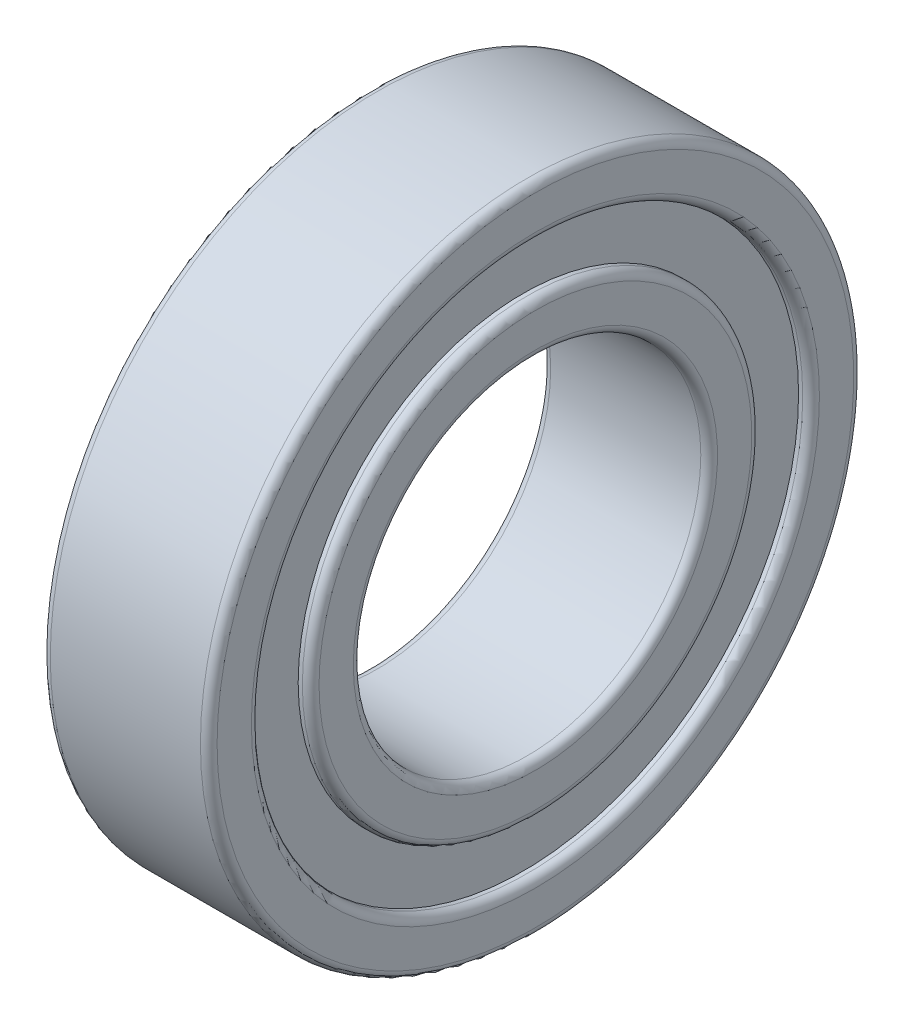
from build123d import *
from build123d.topology import SkipClean

# Parameters (mm, degrees)
SKETCH_5_W               = 1.65
SKETCH_5_H               = 1.1
PATTERN_CIRCULAR_5_COUNT = 16
PATTERN_CIRCULAR_2_COUNT = 16
SKETCH_8_W               = 0.6
SKETCH_8_H               = 4.866666666


with BuildPart() as part:
    # 草图2 → 旋转1 (revolve)
    with BuildSketch(Plane.XY, mode=Mode.PRIVATE) as revolve_1_sk:
        with BuildLine():
            Line((5.4, 12.5), (-5.4, 12.5))
            ThreePointArc((-5.4, 12.5), (-5.824264069, 12.675735931), (-6, 13.1))
            Line((-6, 13.1), (-6, 15.566666667))
            ThreePointArc((-6, 15.566666667), (-5.824264069, 15.990930735), (-5.4, 16.166666667))
            Line((-5.4, 16.166666667), (-2.049728979, 16.166666667))
            ThreePointArc((-2.049728979, 16.166666667), (0, 15.25), (2.049728979, 16.166666667))
            Line((2.049728979, 16.166666667), (5.4, 16.166666667))
            ThreePointArc((5.4, 16.166666667), (5.824264069, 15.990930735), (6, 15.566666667))
            Line((6, 15.566666667), (6, 13.1))
            ThreePointArc((6, 13.1), (5.824264069, 12.675735931), (5.4, 12.5))
        make_face()
        with BuildLine():
            Line((-6, 22.9), (-6, 20.433333333))
            ThreePointArc((-6, 20.433333333), (-5.824264069, 20.009069265), (-5.4, 19.833333333))
            Line((-5.4, 19.833333333), (-2.049728979, 19.833333333))
            ThreePointArc((-2.049728979, 19.833333333), (0, 20.75), (2.049728979, 19.833333333))
            Line((2.049728979, 19.833333333), (5.4, 19.833333333))
            ThreePointArc((5.4, 19.833333333), (5.824264069, 20.009069265), (6, 20.433333333))
            Line((6, 20.433333333), (6, 22.9))
            ThreePointArc((6, 22.9), (5.824264069, 23.324264069), (5.4, 23.5))
            Line((5.4, 23.5), (-5.4, 23.5))
            ThreePointArc((-5.4, 23.5), (-5.824264069, 23.324264069), (-6, 22.9))
        make_face()
    revolve(revolve_1_sk.sketch.rotate(Axis((-3.5, 0, 0), (1, 0, 0)), 90), axis=Axis((-3.5, 0, 0), (1, 0, 0)))


with BuildPart() as body_2:
    # 草图5 → 旋转3 (revolve)
    with BuildSketch(Plane.XY, mode=Mode.PRIVATE) as revolve_3_sk:
        with Locations((0, 18)):
            Rectangle(SKETCH_5_W, SKETCH_5_H)
    revolve(revolve_3_sk.sketch.rotate(Axis((-19.927092192, 0, 0), (1, 0, 0)), 90), axis=Axis((-19.927092192, 0, 0), (1, 0, 0)))



with BuildPart() as body_3:
    # 草图3 → 旋转2 (revolve)
    with BuildSketch(Plane.XY):
        with BuildLine():
            Line((-3.025, 18), (3.025, 18))
            ThreePointArc((3.025, 18), (0, 21.025), (-3.025, 18))
        make_face()
    revolve(axis=Axis((-3.025, 18, 0), (1, 0, 0)))


with BuildPart() as pattern_circular_5_1:
    # 阵列(圆周)5: pattern copy
    add(body_3.part.rotate(Axis((0, 0, 0), (1, 0, 0)), 1 * 360 / PATTERN_CIRCULAR_5_COUNT))


with BuildPart() as pattern_circular_5_2:
    # 阵列(圆周)5: pattern copy
    add(body_3.part.rotate(Axis((0, 0, 0), (1, 0, 0)), 2 * 360 / PATTERN_CIRCULAR_5_COUNT))


with BuildPart() as pattern_circular_5_3:
    # 阵列(圆周)5: pattern copy
    add(body_3.part.rotate(Axis((0, 0, 0), (1, 0, 0)), 3 * 360 / PATTERN_CIRCULAR_5_COUNT))


with BuildPart() as pattern_circular_5_4:
    # 阵列(圆周)5: pattern copy
    add(body_3.part.rotate(Axis((0, 0, 0), (1, 0, 0)), 4 * 360 / PATTERN_CIRCULAR_5_COUNT))


with BuildPart() as pattern_circular_5_5:
    # 阵列(圆周)5: pattern copy
    add(body_3.part.rotate(Axis((0, 0, 0), (1, 0, 0)), 5 * 360 / PATTERN_CIRCULAR_5_COUNT))


with BuildPart() as pattern_circular_5_6:
    # 阵列(圆周)5: pattern copy
    add(body_3.part.rotate(Axis((0, 0, 0), (1, 0, 0)), 6 * 360 / PATTERN_CIRCULAR_5_COUNT))


with BuildPart() as pattern_circular_5_7:
    # 阵列(圆周)5: pattern copy
    add(body_3.part.rotate(Axis((0, 0, 0), (1, 0, 0)), 7 * 360 / PATTERN_CIRCULAR_5_COUNT))


with BuildPart() as pattern_circular_5_8:
    # 阵列(圆周)5: pattern copy
    add(body_3.part.rotate(Axis((0, 0, 0), (1, 0, 0)), 8 * 360 / PATTERN_CIRCULAR_5_COUNT))


with BuildPart() as pattern_circular_5_9:
    # 阵列(圆周)5: pattern copy
    add(body_3.part.rotate(Axis((0, 0, 0), (1, 0, 0)), 9 * 360 / PATTERN_CIRCULAR_5_COUNT))


with BuildPart() as pattern_circular_5_10:
    # 阵列(圆周)5: pattern copy
    add(body_3.part.rotate(Axis((0, 0, 0), (1, 0, 0)), 10 * 360 / PATTERN_CIRCULAR_5_COUNT))


with BuildPart() as pattern_circular_5_11:
    # 阵列(圆周)5: pattern copy
    add(body_3.part.rotate(Axis((0, 0, 0), (1, 0, 0)), 11 * 360 / PATTERN_CIRCULAR_5_COUNT))


with BuildPart() as pattern_circular_5_12:
    # 阵列(圆周)5: pattern copy
    add(body_3.part.rotate(Axis((0, 0, 0), (1, 0, 0)), 12 * 360 / PATTERN_CIRCULAR_5_COUNT))


with BuildPart() as pattern_circular_5_13:
    # 阵列(圆周)5: pattern copy
    add(body_3.part.rotate(Axis((0, 0, 0), (1, 0, 0)), 13 * 360 / PATTERN_CIRCULAR_5_COUNT))


with BuildPart() as pattern_circular_5_14:
    # 阵列(圆周)5: pattern copy
    add(body_3.part.rotate(Axis((0, 0, 0), (1, 0, 0)), 14 * 360 / PATTERN_CIRCULAR_5_COUNT))


with BuildPart() as pattern_circular_5_15:
    # 阵列(圆周)5: pattern copy
    add(body_3.part.rotate(Axis((0, 0, 0), (1, 0, 0)), 15 * 360 / PATTERN_CIRCULAR_5_COUNT))


with BuildPart() as cut_revolve_1_tool:
    # 草图6 → 切除-旋转1 (revolve)
    with BuildSketch(Plane.XY):
        with BuildLine():
            Line((-2.974579802, 18.55), (2.974579802, 18.55))
            ThreePointArc((2.974579802, 18.55), (0, 21.025), (-2.974579802, 18.55))
        make_face()
        with BuildLine():
            Line((-2.974579802, 17.45), (2.974579802, 17.45))
            ThreePointArc((2.974579802, 17.45), (0, 14.975), (-2.974579802, 17.45))
        make_face()
    revolve(axis=Axis((-19.927092192, 0, 0), (1, 0, 0)))


with BuildPart() as part_1:
    add(part.part)

    # 切除-旋转1: cut by cut_revolve_1_tool
    add(cut_revolve_1_tool.part, mode=Mode.SUBTRACT)

    # 草图8 → 旋转5 (revolve)
    with BuildSketch(Plane.XY, mode=Mode.PRIVATE) as revolve_5_sk:
        with Locations((4.8, 18)):
            Rectangle(SKETCH_8_W, SKETCH_8_H)
        with Locations((-4.8, 18)):
            Rectangle(SKETCH_8_W, SKETCH_8_H)
    revolve(revolve_5_sk.sketch.rotate(Axis((-19.927092192, 0, 0), (1, 0, 0)), 90), axis=Axis((-19.927092192, 0, 0), (1, 0, 0)))


with BuildPart() as body_3_1:
    add(body_3.part)

    # 切除-旋转1: cut by cut_revolve_1_tool
    add(cut_revolve_1_tool.part, mode=Mode.SUBTRACT)


with BuildPart() as pattern_circular_5_1_1:
    add(pattern_circular_5_1.part)

    # 切除-旋转1: cut by cut_revolve_1_tool
    add(cut_revolve_1_tool.part, mode=Mode.SUBTRACT)


with BuildPart() as pattern_circular_5_2_1:
    add(pattern_circular_5_2.part)

    # 切除-旋转1: cut by cut_revolve_1_tool
    add(cut_revolve_1_tool.part, mode=Mode.SUBTRACT)


with BuildPart() as pattern_circular_5_3_1:
    add(pattern_circular_5_3.part)

    # 切除-旋转1: cut by cut_revolve_1_tool
    add(cut_revolve_1_tool.part, mode=Mode.SUBTRACT)


with BuildPart() as pattern_circular_5_4_1:
    add(pattern_circular_5_4.part)

    # 切除-旋转1: cut by cut_revolve_1_tool
    add(cut_revolve_1_tool.part, mode=Mode.SUBTRACT)


with BuildPart() as pattern_circular_5_5_1:
    add(pattern_circular_5_5.part)

    # 切除-旋转1: cut by cut_revolve_1_tool
    add(cut_revolve_1_tool.part, mode=Mode.SUBTRACT)


with BuildPart() as pattern_circular_5_6_1:
    add(pattern_circular_5_6.part)

    # 切除-旋转1: cut by cut_revolve_1_tool
    add(cut_revolve_1_tool.part, mode=Mode.SUBTRACT)


with BuildPart() as pattern_circular_5_7_1:
    add(pattern_circular_5_7.part)

    # 切除-旋转1: cut by cut_revolve_1_tool
    add(cut_revolve_1_tool.part, mode=Mode.SUBTRACT)


with BuildPart() as pattern_circular_5_8_1:
    add(pattern_circular_5_8.part)

    # 切除-旋转1: cut by cut_revolve_1_tool
    add(cut_revolve_1_tool.part, mode=Mode.SUBTRACT)


with BuildPart() as pattern_circular_5_9_1:
    add(pattern_circular_5_9.part)

    # 切除-旋转1: cut by cut_revolve_1_tool
    add(cut_revolve_1_tool.part, mode=Mode.SUBTRACT)


with BuildPart() as pattern_circular_5_10_1:
    add(pattern_circular_5_10.part)

    # 切除-旋转1: cut by cut_revolve_1_tool
    add(cut_revolve_1_tool.part, mode=Mode.SUBTRACT)


with BuildPart() as pattern_circular_5_11_1:
    add(pattern_circular_5_11.part)

    # 切除-旋转1: cut by cut_revolve_1_tool
    add(cut_revolve_1_tool.part, mode=Mode.SUBTRACT)


with BuildPart() as pattern_circular_5_12_1:
    add(pattern_circular_5_12.part)

    # 切除-旋转1: cut by cut_revolve_1_tool
    add(cut_revolve_1_tool.part, mode=Mode.SUBTRACT)


with BuildPart() as pattern_circular_5_13_1:
    add(pattern_circular_5_13.part)

    # 切除-旋转1: cut by cut_revolve_1_tool
    add(cut_revolve_1_tool.part, mode=Mode.SUBTRACT)


with BuildPart() as pattern_circular_5_14_1:
    add(pattern_circular_5_14.part)

    # 切除-旋转1: cut by cut_revolve_1_tool
    add(cut_revolve_1_tool.part, mode=Mode.SUBTRACT)


with BuildPart() as pattern_circular_5_15_1:
    add(pattern_circular_5_15.part)

    # 切除-旋转1: cut by cut_revolve_1_tool
    add(cut_revolve_1_tool.part, mode=Mode.SUBTRACT)


with BuildPart() as body_2_1:
    with SkipClean():  # the faces are left unmerged after this step: merging them gives an invalid solid
        add(body_2.part)

        add(body_3_1.part)  # 旋转4 merges body 3
        # 草图7 → 旋转4 (revolve)
        with BuildSketch(Plane.XY):
            with BuildLine():
                Line((-2.75, 18), (2.75, 18))
                ThreePointArc((2.75, 18), (0, 20.75), (-2.75, 18))
            make_face()
        revolve_4 = revolve(axis=Axis((-2.75, 18, 0), (1, 0, 0)))

    # 阵列(圆周)2: 旋转4 ×16 about axis
    pattern_circular_2_axis = Axis((0, 0, 0), (1, 0, 0))
    for i in range(1, PATTERN_CIRCULAR_2_COUNT):
        add(revolve_4.rotate(pattern_circular_2_axis, i * 360 / PATTERN_CIRCULAR_2_COUNT))


solid = Compound([part_1.part, pattern_circular_5_1_1.part, pattern_circular_5_2_1.part, pattern_circular_5_3_1.part, pattern_circular_5_4_1.part, pattern_circular_5_5_1.part, pattern_circular_5_6_1.part, pattern_circular_5_7_1.part, pattern_circular_5_8_1.part, pattern_circular_5_9_1.part, pattern_circular_5_10_1.part, pattern_circular_5_11_1.part, pattern_circular_5_12_1.part, pattern_circular_5_13_1.part, pattern_circular_5_14_1.part, pattern_circular_5_15_1.part, body_2_1.part])
